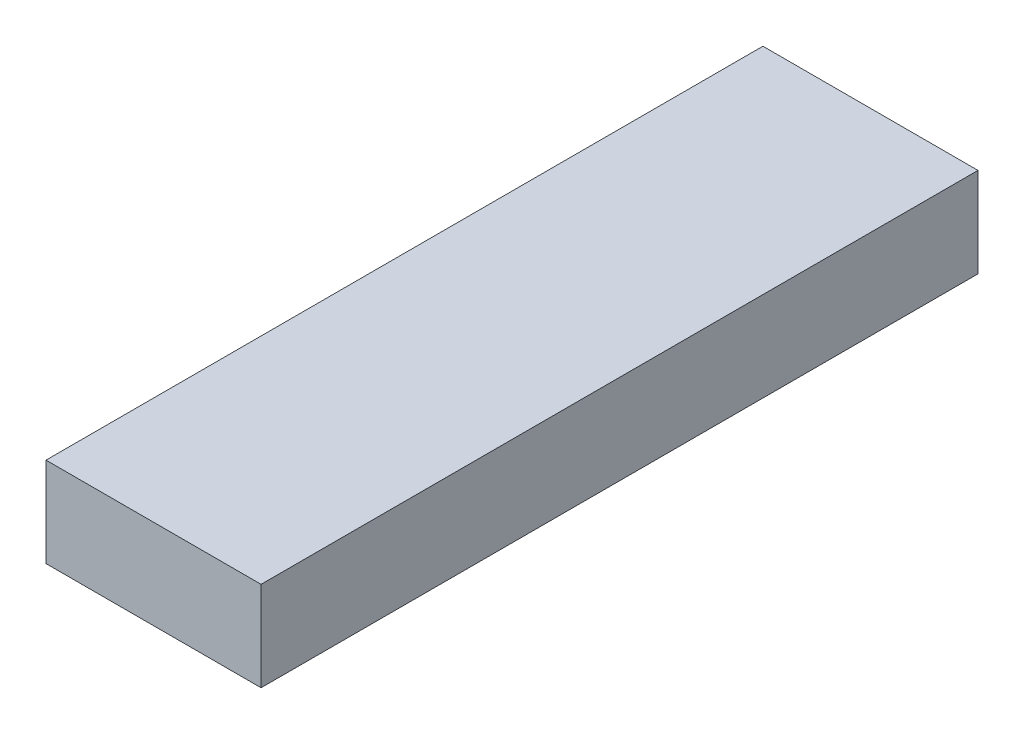
SolidWorks part; units mm, degrees
ref_plane "Front Plane" through (0, 0, 0) normal (0, 0, 1) x (1, 0, 0)
ref_plane "Top Plane" through (0, 0, 0) normal (0, 1, 0) x (1, 0, 0)
ref_plane "Right Plane" through (0, 0, 0) normal (1, 0, 0) x (0, 0, -1)
other "Configuration Table"
sketch "Sketch1" plane through (0, 0, 0) normal (0, 0, 1) x (1, 0, 0)
  line L13 (0, 0) -> (120, 0)
  line L14 (0, 0) -> (0, 50)
  line L15 (0, 50) -> (120, 50)
  line L16 (120, 0) -> (120, 50)
  dimension "D1" = 120
  dimension "D2" = 50
extrude "Boss-Extrude1" add sketch "Sketch1" along normal blind 400
